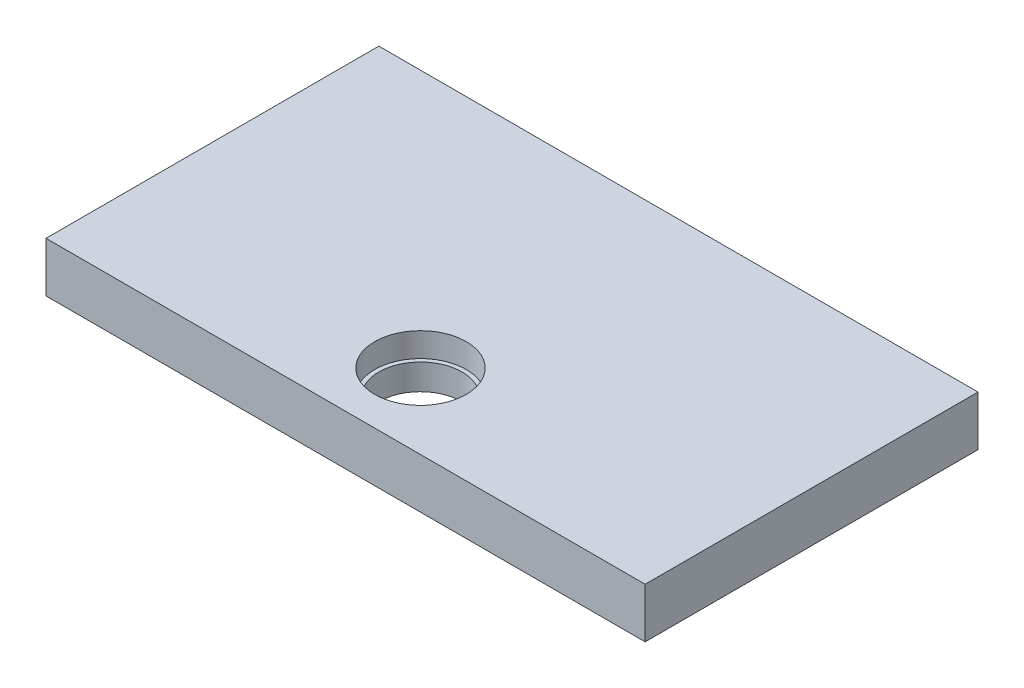
from build123d import *

# Parameters (mm, degrees)
SKETCH_1_W          = 360
SKETCH_1_H          = 200
EXTRUDE_1_DEPTH     = 30
SKETCH_2_R          = 27.5
CUT_EXTRUDE_1_DEPTH = 14.53
SKETCH_3_R          = 25
CUT_EXTRUDE_2_DEPTH = 209.086520467


with BuildPart() as part:
    # 草图1 → 凸台-拉伸1 (new body)
    with BuildSketch(Plane(origin=(0, 0, 0), x_dir=(1, 0, 0), z_dir=(0, 1, 0))):
        Rectangle(SKETCH_1_W, SKETCH_1_H)
    extrude(amount=EXTRUDE_1_DEPTH)

    # 草图2 → 切除-拉伸1 (cut)
    with BuildSketch(Plane(origin=(0, 30, 0), x_dir=(1, 0, 0), z_dir=(0, 1, 0))):
        with Locations(Location((0, -55, 0), (0, 0, 270))):
            Circle(SKETCH_2_R)
    extrude(amount=-CUT_EXTRUDE_1_DEPTH, mode=Mode.SUBTRACT)

    # 草图3 → 切除-拉伸2 (cut, through all)
    with BuildSketch(Plane(origin=(0, 30, 0), x_dir=(1, 0, 0), z_dir=(0, 1, 0))):
        with Locations(Location((0, -55, 0), (0, 0, 270))):
            Circle(SKETCH_3_R)
    extrude(amount=-CUT_EXTRUDE_2_DEPTH, mode=Mode.SUBTRACT)


solid = part.part
